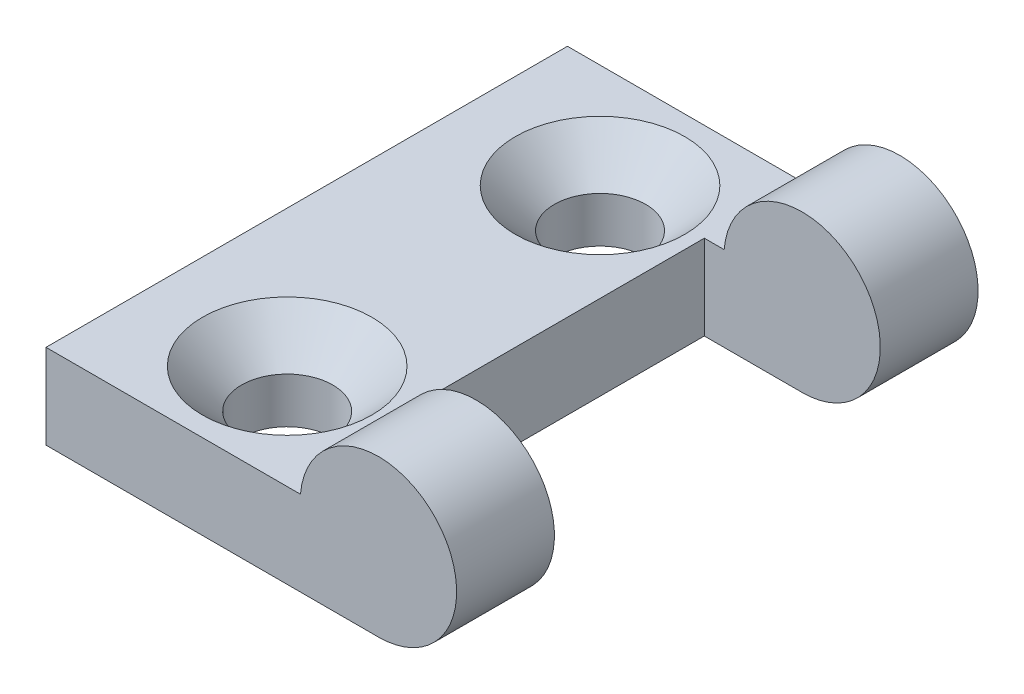
SolidWorks part; units mm, degrees
ref_plane "前视基准面" through (0, 0, 0) normal (0, 0, 1) x (1, 0, 0)
ref_plane "上视基准面" through (0, 0, 0) normal (0, 1, 0) x (1, 0, 0)
ref_plane "右视基准面" through (0, 0, 0) normal (1, 0, 0) x (0, 0, -1)
sketch "草图1" plane through (0, 0, 0) normal (0, 1, 0) x (1, 0, 0)
  line L1 (-12.75, 20) -> (12.75, 20)
  line L2 (-12.75, 20) -> (-12.75, -20)
  line L3 (-12.75, -20) -> (12.75, -20)
  line L4 (12.75, 20) -> (12.75, -20)
  line L5 (-12.75, 20) -> (12.75, -20) construction
  line L6 (-12.75, -20) -> (12.75, 20) construction
  point P0 (0, 0)
  dimension "D1" = 25.5
  dimension "D2" = 40
extrude "凸台-拉伸1" add sketch "草图1" along normal blind 6.5
sketch "草图2" plane through (0, 0, 20) normal (0, 0, 1) x (1, 0, 0)
  line L0 (-12.75, 0) -> (12.75, 0) construction
  line L1 (-12.75, 6.5) -> (-12.75, 0) construction
  circle A0 centre (12.75, 6) radius 6
  dimension "D1" = 25.5
  dimension "D2" = 12
extrude "凸台-拉伸2" add sketch "草图2" against normal up to surface (40 mm away) up to face at (0, 3.25, -20)
sketch "草图3" plane through (0, 0, 0) normal (0, -1, 0) x (1, 0, 0)
  line L0 (18.75, -20) -> (18.75, 20) construction
  line L1 (32.25, -12.5) -> (5.25, -12.5)
  line L2 (32.25, -12.5) -> (32.25, 12.5)
  line L3 (32.25, 12.5) -> (5.25, 12.5)
  line L4 (5.25, -12.5) -> (5.25, 12.5)
  line L5 (32.25, -12.5) -> (5.25, 12.5) construction
  line L6 (32.25, 12.5) -> (5.25, -12.5) construction
  point P0 (18.75, 0)
  dimension "D1" = 25
  dimension "D2" = 27
extrude "切除-拉伸1" cut sketch "草图3" against normal through all
sketch "草图5" plane through (0, 6.5, 0) normal (0, 1, 0) x (1, 0, 0)
  line L0 (5.25, 0) -> (37.6851, 0) construction
  line L1 (5.25, 12.5) -> (5.25, -12.5) construction
  line L2 (37.6851, 20.5307) -> (37.6851, -20.5307) construction
  line L3 (-2.25, 12) -> (-2.25, -12) construction
  line L4 (12.75, 20) -> (12.75, 2.5966) construction
  circle A0 centre (-2.25, 12) radius 3.5
  circle A1 centre (-2.25, -12) radius 3.5
  dimension "D3" = 7
  dimension "D1" = 24
  dimension "D2" = 15
extrude "切除-拉伸2" cut sketch "草图5" against normal through all
chamfer "倒角1" distance 3 angle 45 2 edges at (-2.25, 6.5, 15.5) (-2.25, 6.5, -8.5)
